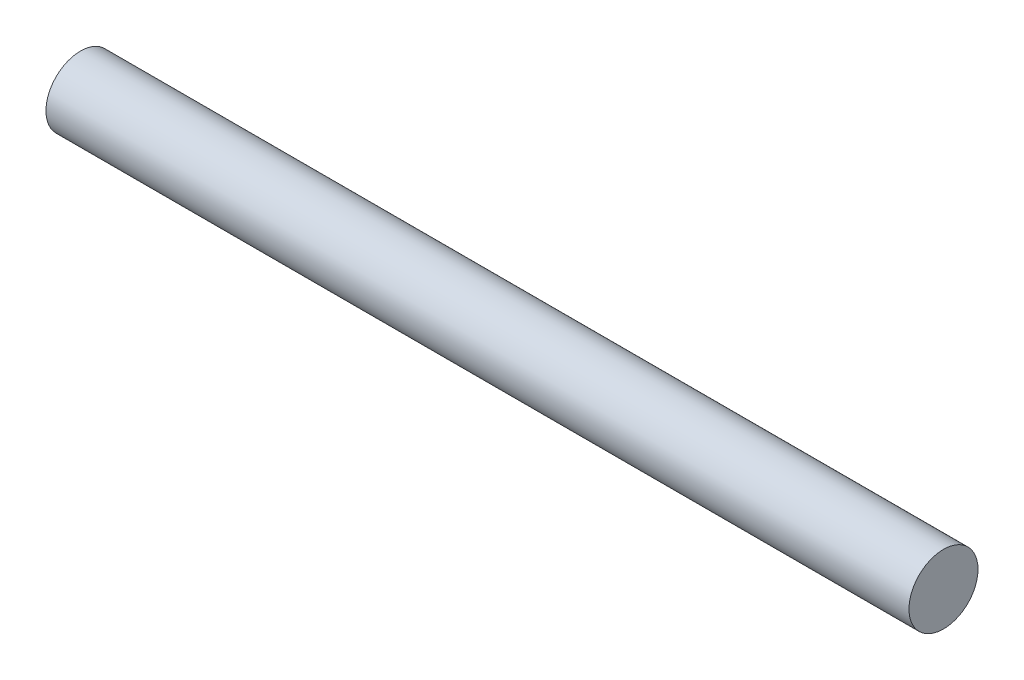
SolidWorks part; units mm, degrees
ref_plane "Front Plane" through (0, 0, 0) normal (0, 0, 1) x (1, 0, 0)
ref_plane "Top Plane" through (0, 0, 0) normal (0, 1, 0) x (1, 0, 0)
ref_plane "Right Plane" through (0, 0, 0) normal (1, 0, 0) x (0, 0, -1)
sketch "Sketch1" plane through (0, 0, 0) normal (1, 0, 0) x (0, 0, -1)
  circle A0 centre (0, 0) radius 20
  dimension "Durchmesser" = 40
extrude "Length" add sketch "Sketch1" along normal blind 500
